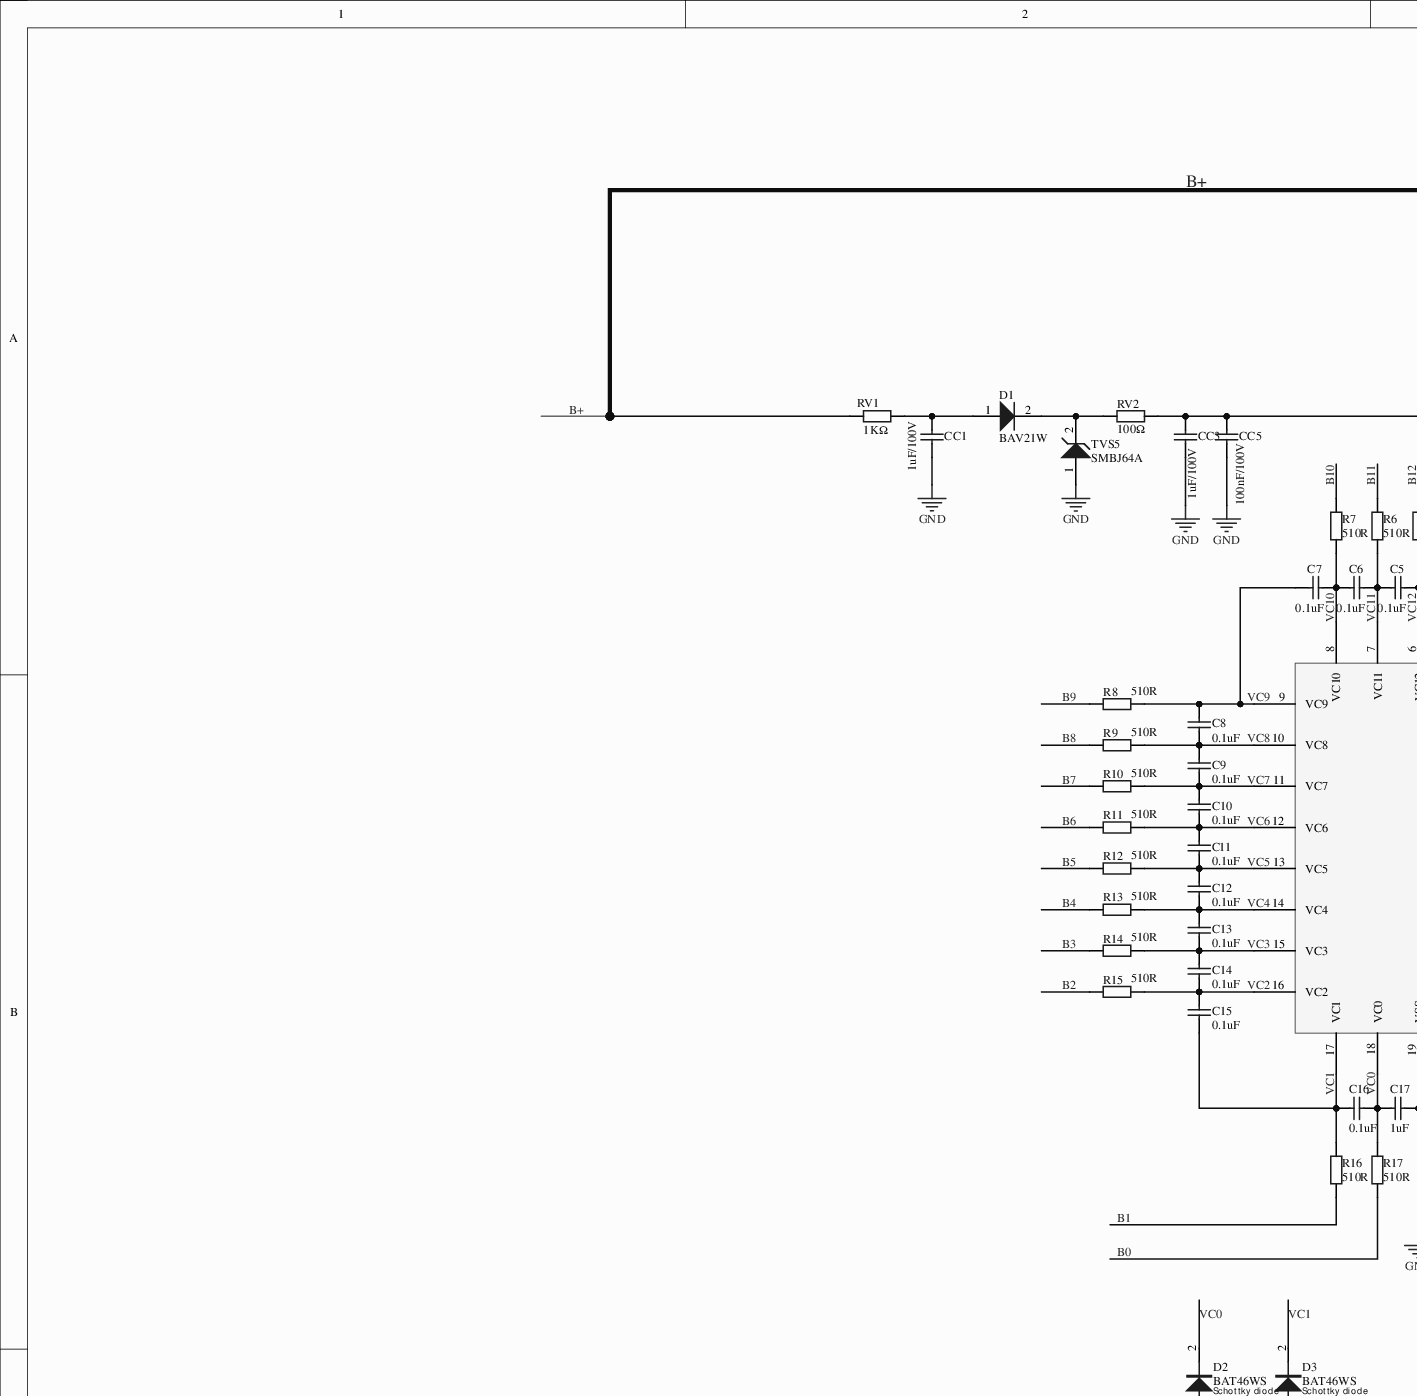
[diagram p0: MISC84412-5.SchDoc, top left]
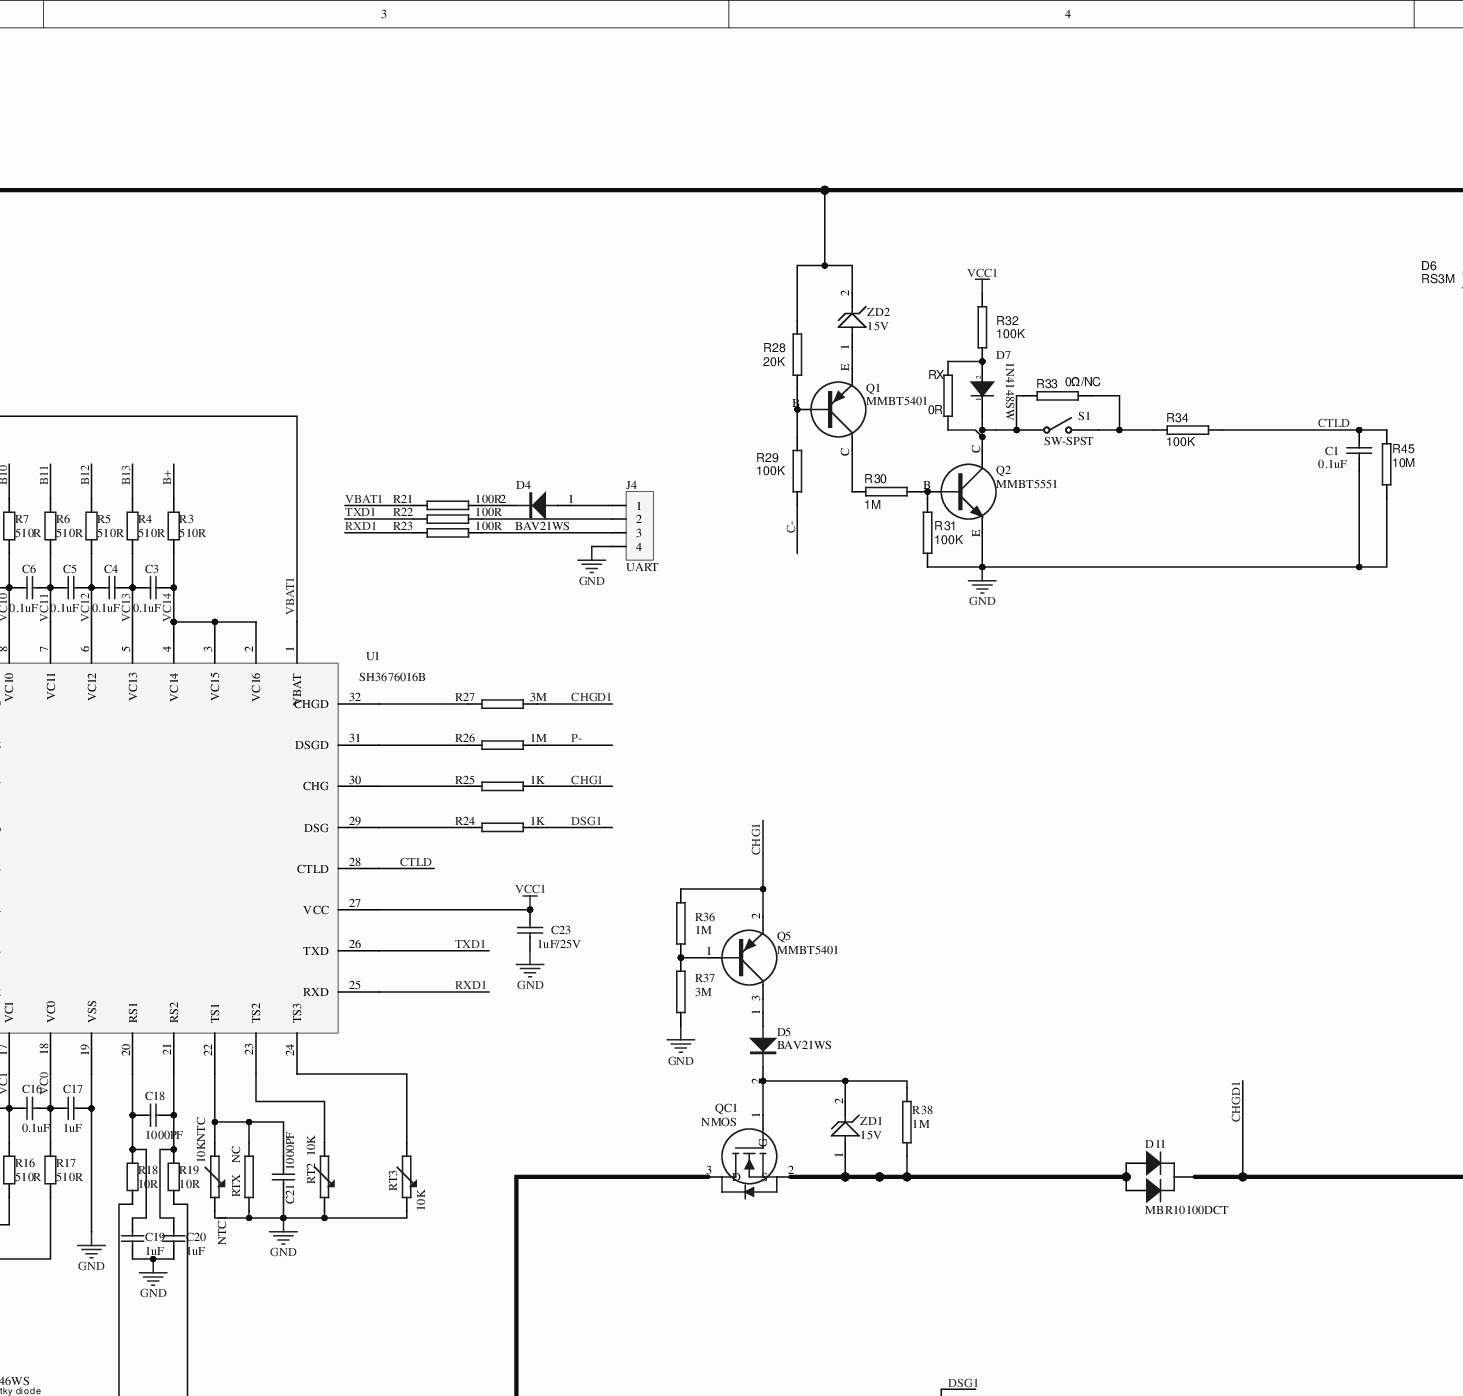
[diagram p1: MISC84412-5.SchDoc, top middle]
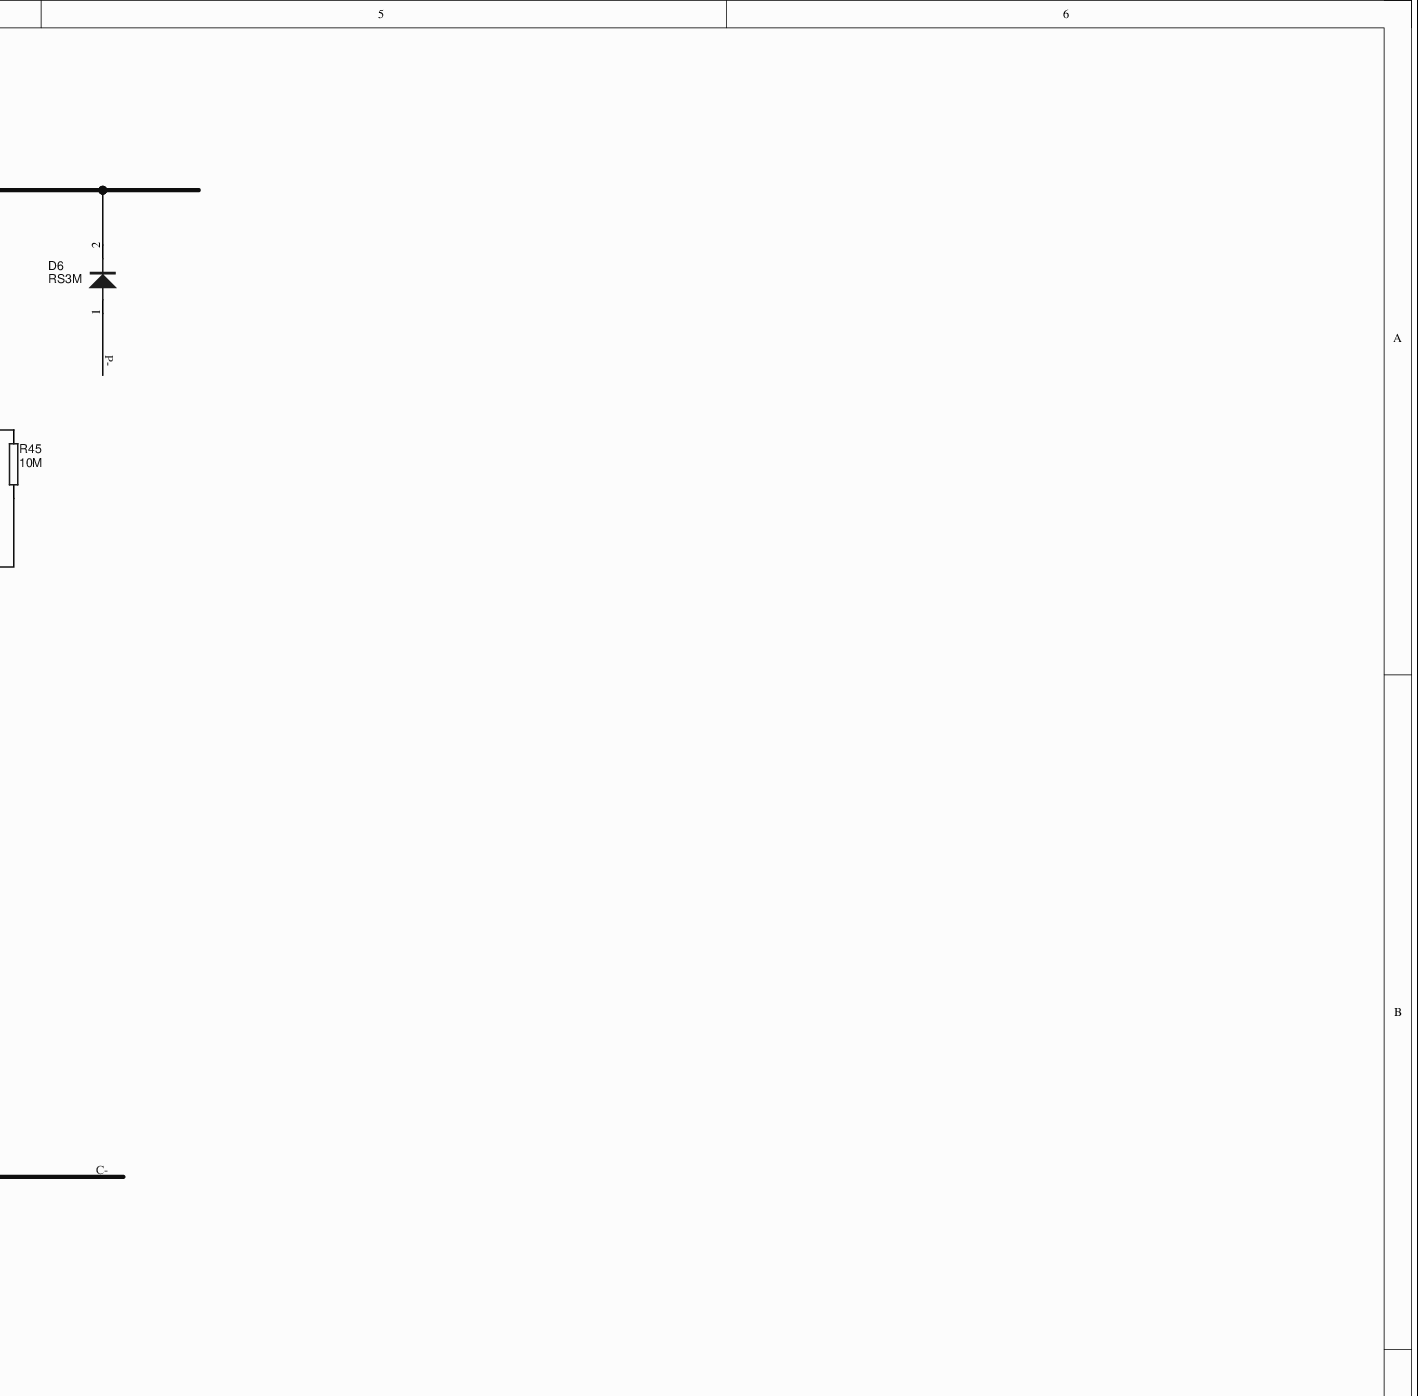
[diagram p2: MISC84412-5.SchDoc, top right]
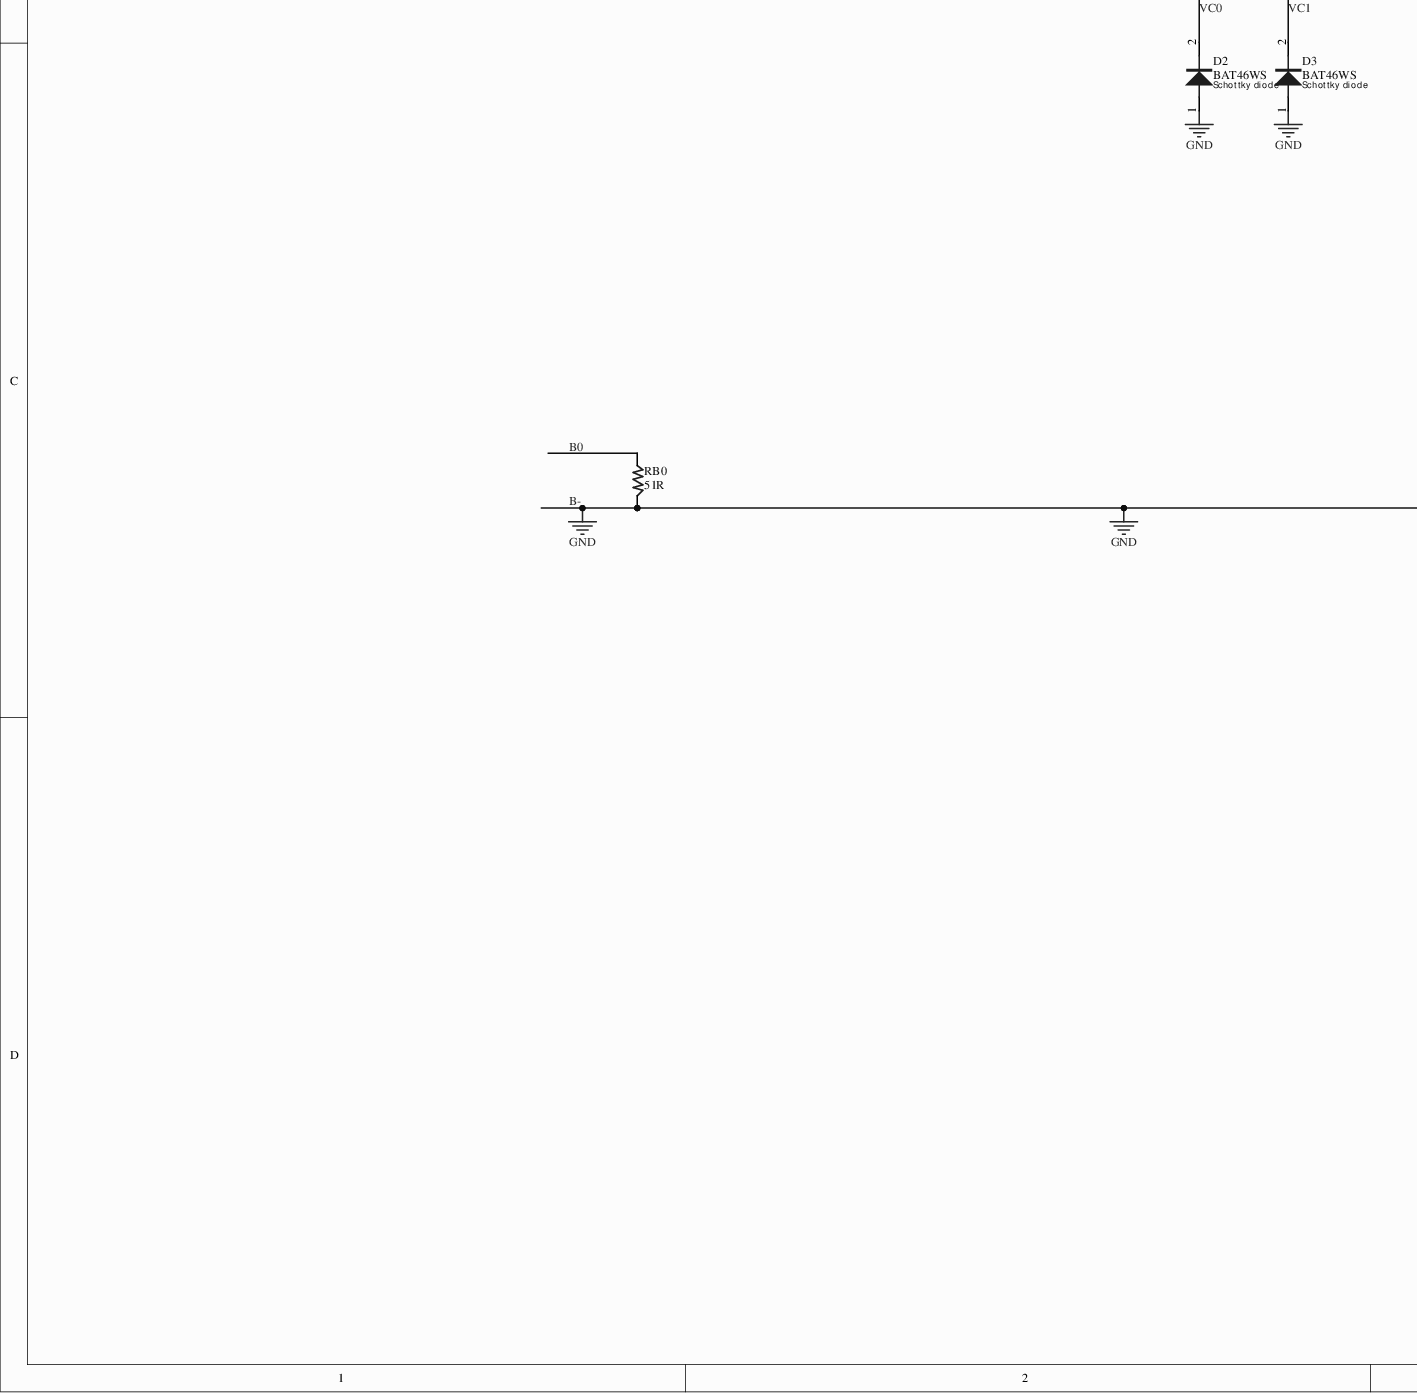
[diagram p3: MISC84412-5.SchDoc, bottom left]
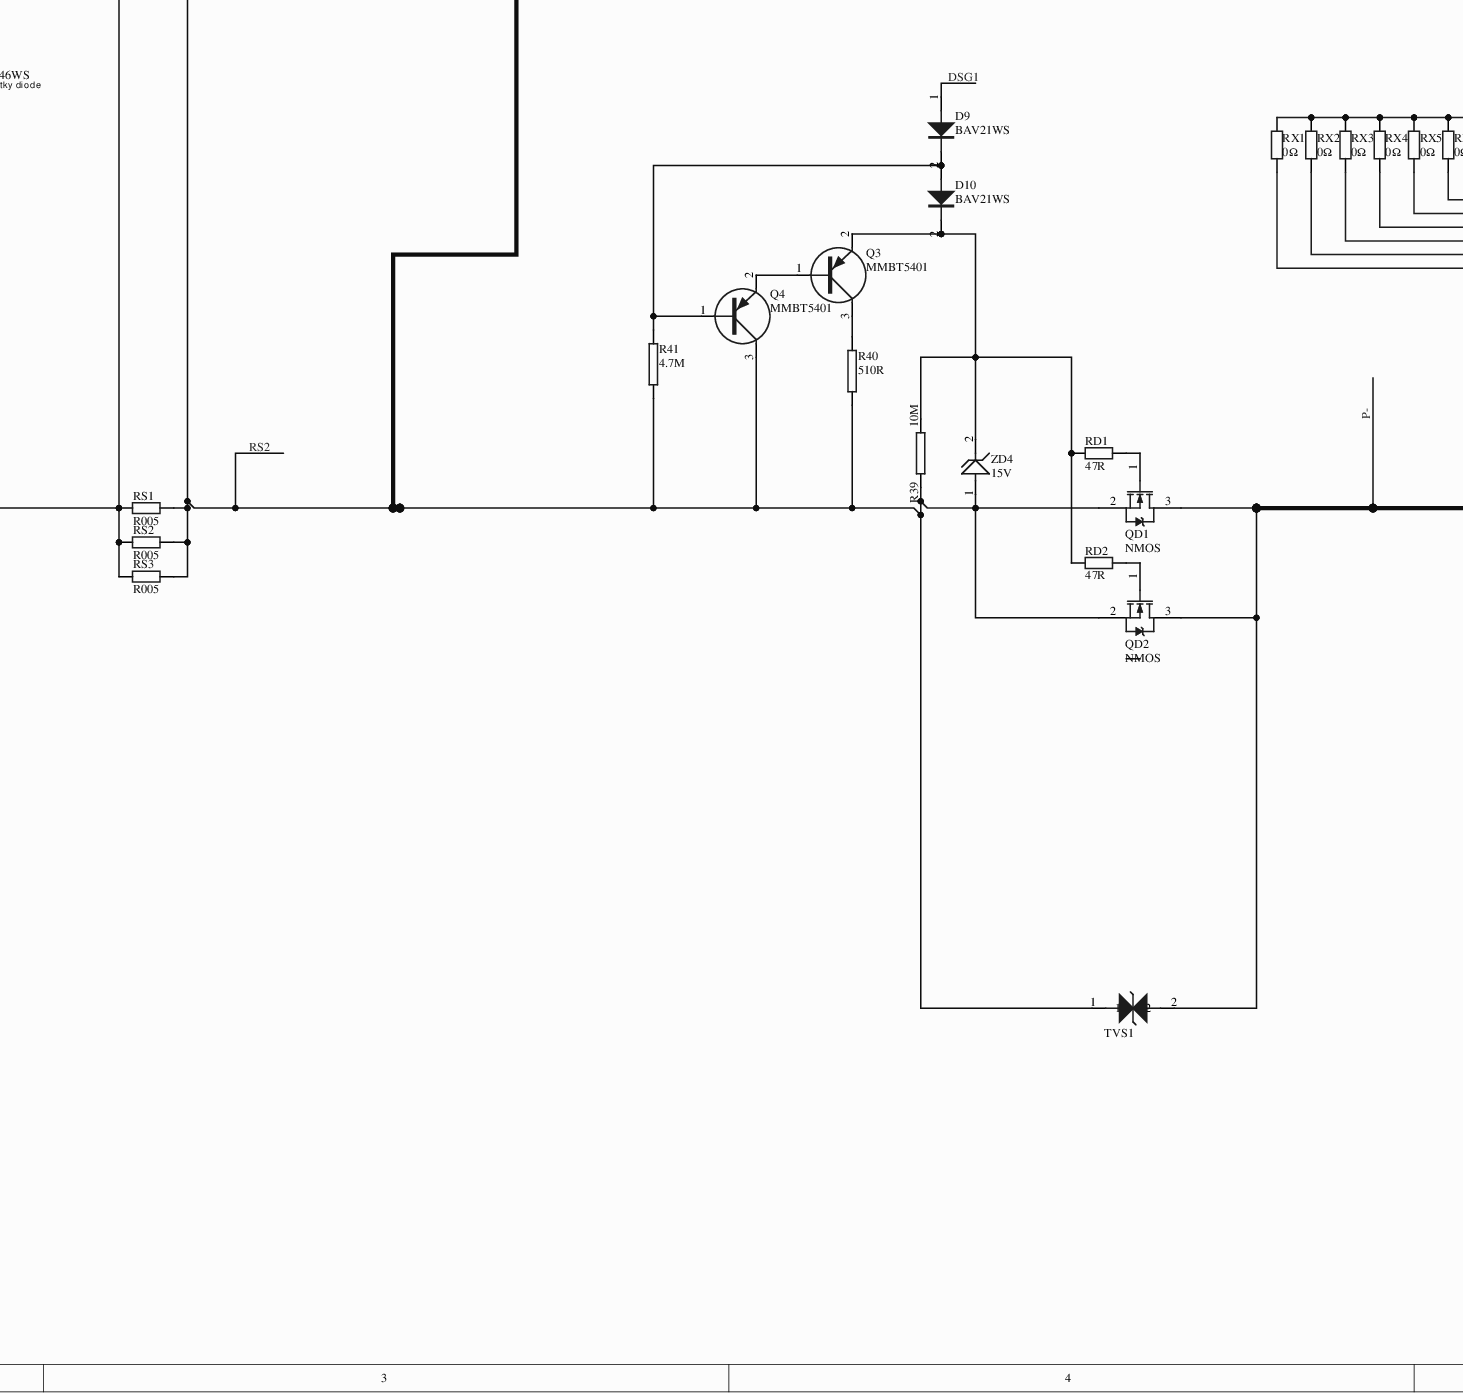
[diagram p4: MISC84412-5.SchDoc, bottom middle]
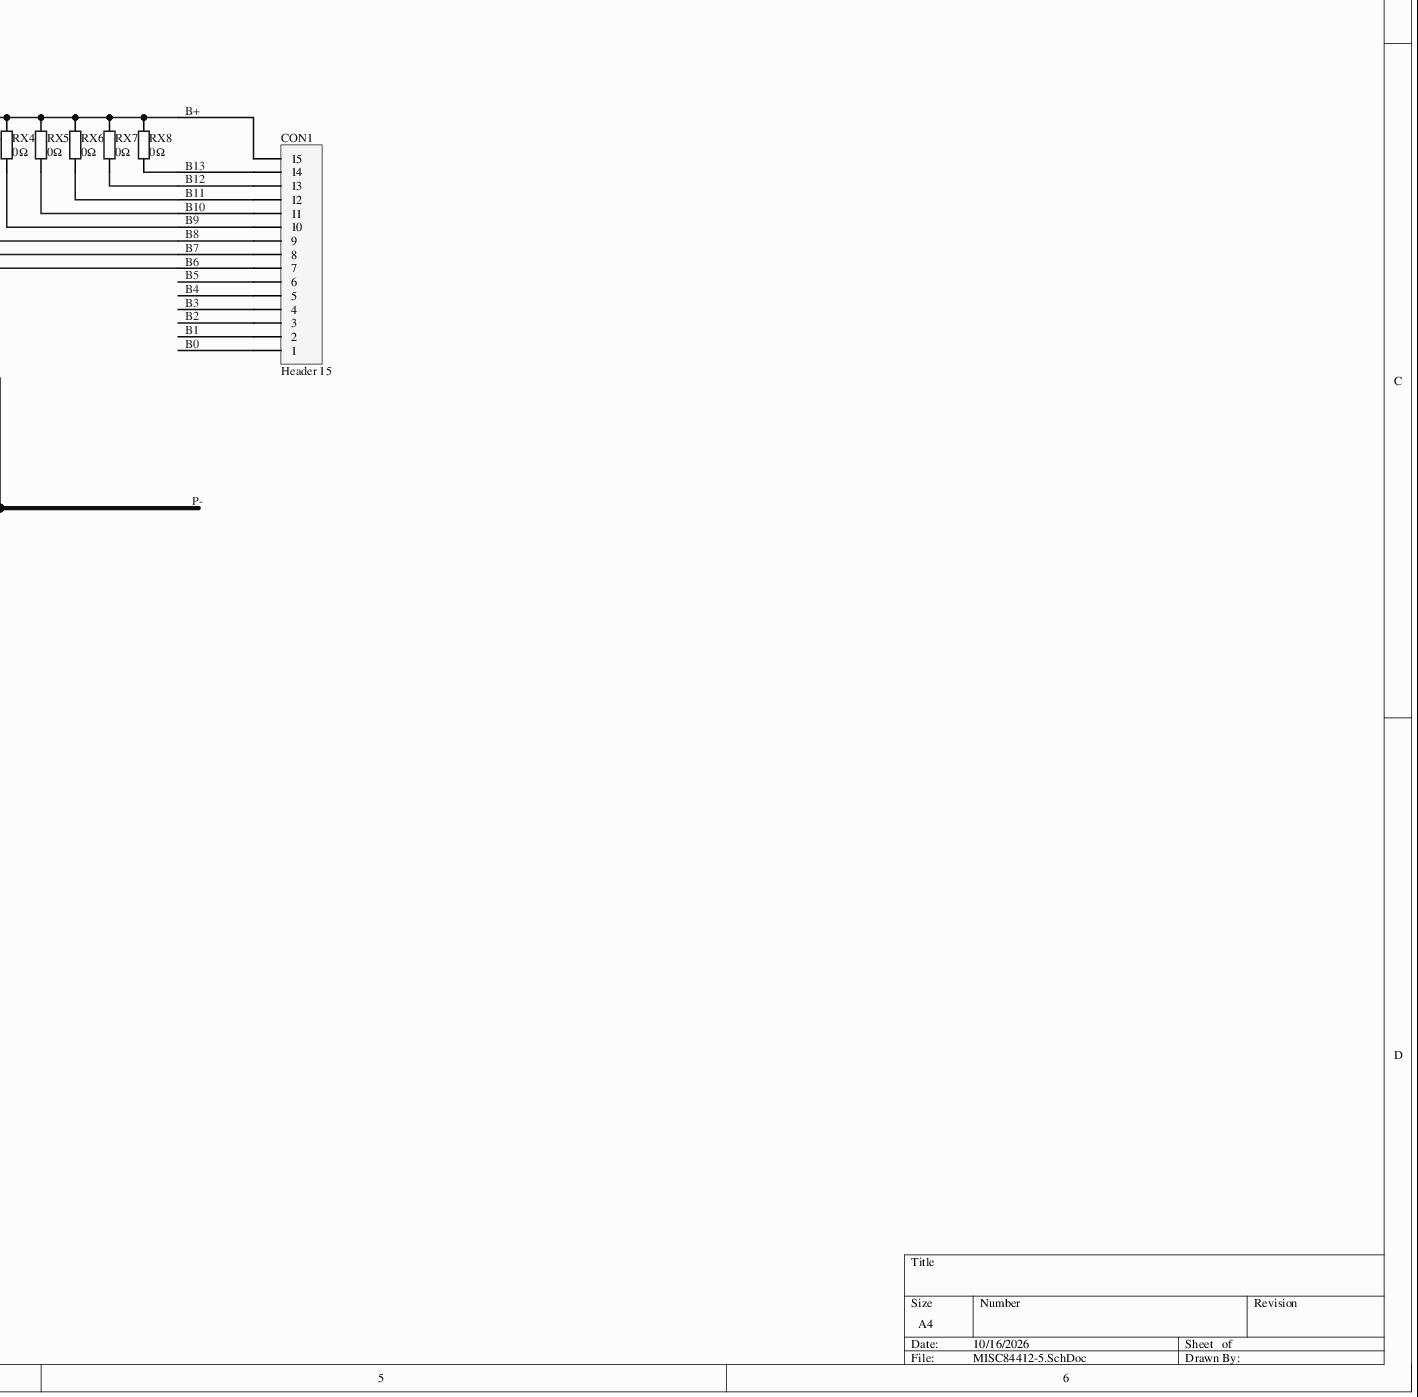
[diagram p5: MISC84412-5.SchDoc, bottom right]
# Altium project MISC84412-3.PrjPcb
1 sheet, 110 parts. Net scope: global (net labels, ports and power ports of the same name join across sheets).
Board file: MISC84412.PcbDoc

## Sheet MISC84412-5.SchDoc
size 762 x 500 mm; SheetNumber: 1; SheetTotal: 1

### Parts
C1  0.1uF  [C0603A]
C3  0.1uF  [C0402A]
C4  0.1uF  [C0402A]
C5  0.1uF  [C0402A]
C6  0.1uF  [C0402A]
C7  0.1uF  [C0402A]
C8  0.1uF  [C0402A]
C9  0.1uF  [C0402A]
C10  0.1uF  [C0402A]
C11  0.1uF  [C0402A]
C12  0.1uF  [C0402A]
C13  0.1uF  [C0402A]
C14  0.1uF  [C0402A]
C15  0.1uF  [C0402A]
C16  0.1uF  [C0402A]
C17  1uF  [C0402A]
C18  1000PF  [C0402A]
C19  1uF  [C0402A]
C20  1uF  [C0402A]
C21  1000PF  [C0603A]
C23  1uF/25V  [C0603A]
CC1  1uF/100V  [C0805L]
CC3  1uF/100V  [C0805L]
CC5  100nF/100V  [C0603A]
CON1  Header 15  [PH-2.0mm15P弯脚不带扣]
D1  BAV21W  [SOD323(1+2-)]
D2  BAT46WS  [SOD323(1+2-)]
D3  BAT46WS  [SOD323(1+2-)]
D4  BAV21WS  [SOD323(1+2-)]
D5  BAV21WS  [SOD323(1+2-)]
D6  RS3M  [SMB M(1+2-)]
D7  1N4148SW  [SOD323]
D9  BAV21WS  [SOD323(1+2-)]
D10  BAV21WS  [SOD323(1+2-)]
D11  MBR10100DCT  [TO-252-DIODE-DUAL]
J4  UART  [CH-2.0-4P]
NTC1  10KNTC  [RT2.3X1-2]
Q1  MMBT5401  [SOT23-3_BEC]
Q2  MMBT5551  [SOT23-3_BEC]
Q3  MMBT5401  [SOT23-3]
Q4  MMBT5401  [SOT23-3]
Q5  MMBT5401  [SOT23-3]
QC1  NMOS  [TO-252-DFN]
QD1  NMOS  [TOLL]
QD2  NMOS  [TOLL]
R3  510R  [R0402A]
R4  510R  [R0402A]
R5  510R  [R0402A]
R6  510R  [R0402A]
R7  510R  [R0402A]
R8  510R  [R0402A]
R9  510R  [R0402A]
R10  510R  [R0402A]
R11  510R  [R0402A]
R12  510R  [R0402A]
R13  510R  [R0402A]
R14  510R  [R0402A]
R15  510R  [R0402A]
R16  510R  [R0402A]
R17  510R  [R0402A]
R18  10R  [R0402A]
R19  10R  [R0402A]
R21  100R  [R0402A]
R22  100R  [R0402A]
R23  100R  [R0402A]
R24  1K  [R0603A]
R25  1K  [R0603A]
R26  1M  [R0603A]
R27  3M  [R0603A]
R28  20K  [R0603A]
R29  100K  [R0603A]
R30  1M  [R0603A]
R31  100K  [R0603A]
R32  100K  [R0603A]
R33  0Ω/NC  [R0603A]
R34  100K  [R0603A]
R36  1M  [R0603A]
R37  3M  [R0603A]
R38  1M  [R0603A]
R39  10M  [R0402A]
R40  510R  [R0603A]
R41  4.7M  [R0603A]
R45  10M  [R0603A]
RB0  51R  [R0805L]
RD1  47R  [R0603Ap]
RD2  47R  [R0603Ap]
RS1  R005  [R2512L]
RS2  R005  [R2512L]
RS3  R005  [R2512L]
RT2  10K  [R0603A]
RT3  10K  [R0603A]
RTX  NC  [R0603A]
RV1  1KΩ  [R0805L]
RV2  100Ω  [R0805L]
RX  0R  [R0603A]
RX1  0Ω  [R0805L]
RX2  0Ω  [R0805L]
RX3  0Ω  [R0805L]
RX4  0Ω  [R0805L]
RX5  0Ω  [R0805L]
RX6  0Ω  [R0805L]
RX7  0Ω  [R0805L]
RX8  0Ω  [R0805L]
S1  SW-SPST  [RT2.3X1.2-2]
TVS1  75CA  [SMC_M(DO-214AB)]  (value not drawn)
TVS5  SMBJ64A  [SMB M(1+2-)]
U1  SH3676016B  [LQFP32L(PIN间距0.8mm)]
ZD1  15V  [SOD323(1+2-)]
ZD2  15V  [SOD323(1+2-)]
ZD4  15V  [SOD323(1+2-)]

### Nets
B-: C1.2 C17.1 C19.2 C20.2 C21.2 C23.1 CC1.1 CC3.1 CC5.1 D2.1(A) D3.1(A) J4.4 NTC1.2 Q2.E R18.2 R31.1 R37.2 R45.2 RB0.1 RS1.1 RS2.1 RS3.1 RT2.2 RT3.2 RTX.2 TVS5.1(A) U1.19(VSS)  [also labelled GND]
VCC1: C23.2 R32.1 U1.27(VCC)
B0: CON1.1 R17.2 RB0.2
B1: CON1.2 R16.2
B2: CON1.3 R15.1
B3: CON1.4 R14.2
B4: CON1.5 R13.2
B5: CON1.6 R12.2
B6: CON1.7 R11.2 RX1.2
B7: CON1.8 R10.2 RX2.2
B8: CON1.9 R9.2 RX3.2
B9: CON1.10 R8.2 RX4.2
B10: CON1.11 R7.2 RX5.2
B11: CON1.12 R6.2 RX6.2
B12: CON1.13 R5.2 RX7.2
B13: CON1.14 R4.2 RX8.2
B+: CON1.15 D6.2(K) R3.2 R28.2 RV1.2 RX1.1 RX2.1 RX3.1 RX4.1 RX5.1 RX6.1 RX7.1 RX8.1 ZD2.2
C-: D11.3(K) R27.1 R29.1  [also labelled CHGD1]
CHG1: Q5.2 R25.1 R36.2
CTLD: C1.1 R34.2 R45.1 U1.28(CTLD)
DSG1: D9.1(A) R24.1
P-: D6.1(A) QD1.3(D) QD2.3(D) R26.1 TVS1.2
RS2: Q4.3 QC1.3(D) QD1.2(S) QD2.2(S) R19.2 R39.1 R40.2 R41.1 RS1.2 RS2.2 RS3.2 TVS1.1 ZD4.1
RXD1: R23.2 U1.25(RXD)
TXD1: R22.2 U1.26(TXD)
VBAT1: CC3.2 CC5.2 R21.2 RV2.1 U1.1(VBAT)
VC0: C16.1 C17.2 D2.2(K) R17.1 U1.18(VC0)
VC1: C15.1 C16.2 D3.2(K) R16.1 U1.17(VC1)
VC2: C14.1 C15.2 R15.2 U1.16(VC2)
VC3: C13.1 C14.2 R14.1 U1.15(VC3)
VC4: C12.1 C13.2 R13.1 U1.14(VC4)
VC5: C11.1 C12.2 R12.1 U1.13(VC5)
VC6: C10.1 C11.2 R11.1 U1.12(VC6)
VC7: C9.1 C10.2 R10.1 U1.11(VC7)
VC8: C8.1 C9.2 R9.1 U1.10(VC8)
VC9: C7.1 C8.2 R8.1 U1.9(VC9)
VC10: C6.1 C7.2 R7.1 U1.8(VC10)
VC11: C5.1 C6.2 R6.1 U1.7(VC11)
VC12: C4.1 C5.2 R5.1 U1.6(VC12)
VC13: C3.1 C4.2 R4.1 U1.5(VC13)
VC14: C3.2 R3.1 U1.2(VC16) U1.3(VC15) U1.4(VC14)
NetC18_1: C18.1 C20.1 R19.1 U1.21(RS2)
NetC18_2: C18.2 C19.1 R18.1 U1.20(RS1)
NetC21_1: C21.1 NTC1.1 RTX.1 U1.22(TS1)
NetCC1_2: CC1.2 D1.1(A) RV1.1
NetD1_2: D1.2(K) RV2.2 TVS5.2(K)
NetD4_1: D4.1(A) J4.1
NetD4_2: D4.2(K) R21.1
NetD5_1: D5.1(A) Q5.3
NetD5_2: D5.2(K) QC1.1(G) R38.2 ZD1.2
NetD7_1: D7.1(A) Q2.C R33.2 RX.1 S1.1(COMMON)
NetD7_2: D7.2 R32.2 RX.2
NetD9_2: D9.2(K) D10.1(A) Q4.1 R41.2
NetD10_2: D10.2(K) Q3.2 R39.2 RD1.1 RD2.1 ZD4.2
NetD11_1: D11.1(A) D11.2(A) QC1.2(S) R38.1 ZD1.1
NetJ4_2: J4.2 R22.1
NetJ4_3: J4.3 R23.1
NetQ1_B: Q1.B R28.1 R29.2
NetQ1_C: Q1.C R30.2
NetQ1_E: Q1.E ZD2.1
NetQ2_B: Q2.B R30.1 R31.2
NetQ3_1: Q3.1 Q4.2
NetQ3_3: Q3.3 R40.1
NetQ5_1: Q5.1 R36.1 R37.1
NetQD1_1: QD1.1(G) RD1.2
NetQD2_1: QD2.1(G) RD2.2
NetR24_2: R24.2 U1.29(DSG)
NetR25_2: R25.2 U1.30(CHG)
NetR26_2: R26.2 U1.31(DSGD)
NetR27_2: R27.2 U1.32(CHGD)
NetR33_1: R33.1 R34.1 S1.2(NO)
NetRT2_1: RT2.1 U1.23(TS2)
NetRT3_1: RT3.1 U1.24(TS3)

### Notes on the sheet
- (near D3) Schottky diode

### Library data of the parts
C1 C23 = CAP
C3-C21 CC1 CC3 CC5 = 0805 100nF(104) 10% 50V: SMD capacitor; ComponentLink1Description: Supplier link; ComponentLink1URL: http://www.szlcsc.com/product/details_50686.html; Package: 0805; Supplier: LC; SuppliersPartNumber: C49678
CON1 = Header 15: Header15; LatestRevisionDate: 17-Jul-2002; LatestRevisionNote: Re-released for DXP Platform.; Publisher: Altium Limited
D1 = SOD-323 1N4148WS T4: Diode; ComponentLink1Description: Supplier link; ComponentLink1URL: http://www.szlcsc.com/product/details_2485.html; Package: SOD-323; Supplier: LC; SuppliersPartNumber: C2128
D2-D6 D9 D10 = DIODE
D7 = 1N4148SW: SMD diode
D11 = MBR10100DCT: SMD dual diode, common cathode
J4 = CON4
NTC1 RT2 RT3 = RES2: RES
Q1 = PNP: PNP Transistor
Q2 = NPN: NPN Transistor
Q3-Q5 = 8550: PNP
QC1 = MOSFET-N
QD1 QD2 = IRFR014: HEXFET N-Channel Power MOSFET; Note: Pin 2 is trimmed and is electrically connected to Drain.; Value: 60V75A@0.94; Published: 8-Jun-2000; LatestRevisionDate: 17-Jul-2002; LatestRevisionNote: Re-released for DXP Platform.; DatasheetVersion: PD-9.7014; PackageVersion: Feb-2003; PackageReference: TO-252AA; PackageDescription: D-PAK/TO-252-AA; 3 Leads (1 Cropped); Body 10.4 (inc. leads) x 6.7 mm (LxW max); Code_JEDEC: TO-252-AA; ComponentLink1Description: Manufacturer Link; ComponentLink1URL: http://www.irf.com/; ComponentLink2Description: Datasheet; ComponentLink2URL: http://www.irf.com/product-info/datasheets/data/irfr014.pdf; Publisher: Altium Limited
R3-R19 RS1-RS3 = 0603 1KΩ (1001) 1%: SMD resistor; ComponentLink1Description: Supplier link; ComponentLink1URL: http://www.szlcsc.com/product/details_21904.html; Package: 0603; Supplier: LC; SuppliersPartNumber: C21190
R21-R34 R36-R41 R45 RTX RX = RES1: RES
RB0 = RES1: ±5% /UniOhm/yageo/TA-I/Walsin/Ralec
RD1 RD2 = 0603 1.2MΩ (1204) 1%: SMD resistor; ComponentLink1Description: Supplier link; ComponentLink1URL: http://www.szlcsc.com/product/details_23493.html; Package: 0603; Supplier: LC; SuppliersPartNumber: C22766
RV1 RV2 RX1-RX8 = 0805 300Ω (3000) 1%: SMD resistor; ComponentLink1Description: Supplier link; ComponentLink1URL: http://www.szlcsc.com/product/details_18305.html; Package: 0805; Supplier: LC; SuppliersPartNumber: C17617
S1 = SW-SPST: Single-Pole, Single-Throw Switch; Published: 24-Mar-1999; LatestRevisionDate: 17-Jul-2002; LatestRevisionNote: Re-released for DXP Platform.; PackageReference: SPST-2; PackageDescription: Switch; 2 Leads; Publisher: Altium Limited
TVS1 = TVS
TVS5 = LL-34 ZMM5V6: Zener diode; ComponentLink1Description: Supplier link; ComponentLink1URL: http://www.szlcsc.com/product/details_8541.html; Package: LL-34; Supplier: LC; SuppliersPartNumber: C8062
ZD1 ZD2 ZD4 = ZENOR